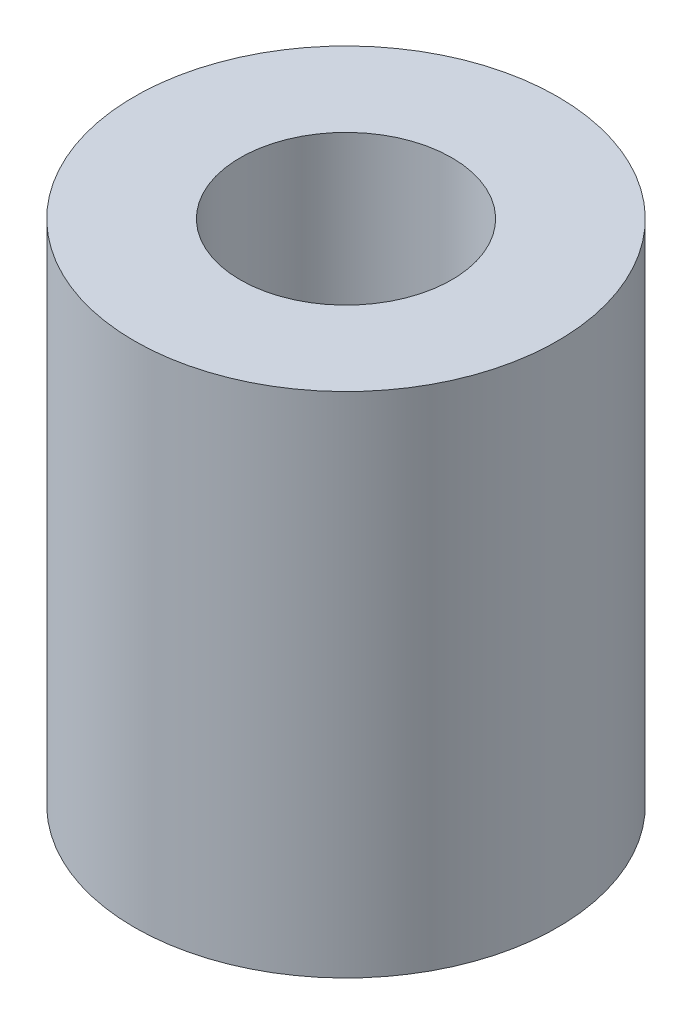
SolidWorks part; units mm, degrees
material "6061 合金"
ref_plane "前视基准面" through (0, 0, 0) normal (0, 0, 1) x (1, 0, 0)
ref_plane "上视基准面" through (0, 0, 0) normal (0, 1, 0) x (1, 0, 0)
ref_plane "右视基准面" through (0, 0, 0) normal (1, 0, 0) x (0, 0, -1)
sketch "草图1" plane through (0, 0, 0) normal (0, 1, 0) x (1, 0, 0)
  circle A0 centre (0, 0) radius 2.5
  dimension "D1" = 5
extrude "凸台-拉伸1" add sketch "草图1" along normal blind 6
sketch "草图2" plane through (0, 6, 0) normal (0, 1, 0) x (1, 0, 0)
  point P0 (0, 0)
hole_wizard "M3 螺纹孔1" positions "草图2" profile "草图3" tap size "M3" standard "GB" end condition through all
sketch "草图3" plane through (0, 6, 0) normal (1, 0, 0) x (0, 0, 1)
  line L0 (0, 0) -> (0, 6)
  line L1 (0, 6) -> (1.25, 6)
  line L2 (1.25, 6) -> (1.25, 0)
  line L5 (1.25, 0) -> (0, 0)
  line L11 (0, -6.35) -> (0, 107.95) construction
  dimension "通孔螺纹孔钻头直径" = 2.5
  dimension "通孔螺纹孔钻头深度" = 6
cosmetic thread "孔螺纹线1" parameters "D2"=3
